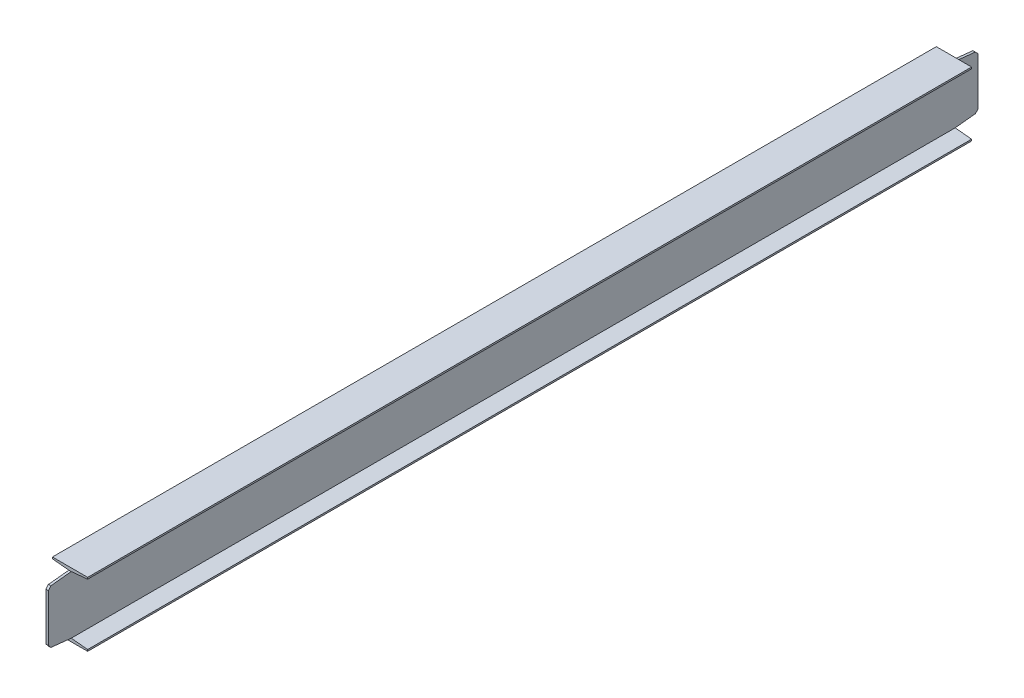
SolidWorks part; units mm, degrees
material "A3"
ref_plane "前视基准面" through (0, 0, 0) normal (0, 0, 1) x (1, 0, 0)
ref_plane "上视基准面" through (0, 0, 0) normal (0, 1, 0) x (1, 0, 0)
ref_plane "右视基准面" through (0, 0, 0) normal (1, 0, 0) x (0, 0, -1)
sketch "草图1" plane through (0, 0, 0) normal (0, 0, 1) x (1, 0, 0)
  line L0 (0, 80) -> (0, -80) construction
  line L1 (9.8926, 0) -> (-9.8926, 0) construction
  line L2 (44, 80) -> (-44, 80)
  line L3 (-44, 80) -> (-44, 76)
  line L4 (-44, 76) -> (-3, 72)
  line L5 (-3, 72) -> (-3, -72)
  line L6 (3, 72) -> (3, -72)
  line L7 (44, 76) -> (3, 72)
  line L8 (44, 80) -> (44, 76)
  line L9 (44, -80) -> (44, -76)
  line L10 (44, -76) -> (3, -72)
  line L11 (-44, -76) -> (-3, -72)
  line L12 (-44, -80) -> (-44, -76)
  line L13 (44, -80) -> (-44, -80)
  point P15 (0, 0)
  point P18 (3, 0)
  point P19 (-3, 0)
  dimension "D1" = 44
  dimension "D2" = 6
  dimension "D3" = 160
  dimension "D4" = 4
  dimension "D5" = 144
extrude "凸台-拉伸1" add sketch "草图1" along normal mid plane 2320
sketch "草图3" plane through (0, 0, 0) normal (1, 0, 0) x (0, 0, -1)
  line L0 (-1160, 66) -> (-1103, 72)
  line L1 (-1160, -72) -> (-1160, 72) construction
  line L2 (-1160, 72) -> (1160, 72) construction
  line L3 (-1103, 72) -> (-1103, 80)
  line L4 (-1160, 80) -> (1160, 80) construction
  line L5 (-1103, 80) -> (-1160, 80)
  line L6 (-1160, 80) -> (-1160, 66)
  line L7 (0, 0) -> (0, 80) construction
  line L8 (1160, 80) -> (1160, 66)
  line L9 (1103, 80) -> (1160, 80)
  line L10 (1103, 72) -> (1103, 80)
  line L11 (1160, 66) -> (1103, 72)
  line L12 (0, 0) -> (1160, 0) construction
  line L13 (1160, -72) -> (1160, 72) construction
  line L14 (1160, -66) -> (1103, -72)
  line L15 (1103, -72) -> (1103, -80)
  line L16 (1103, -80) -> (1160, -80)
  line L17 (1160, -80) -> (1160, -66)
  line L18 (-1160, -80) -> (-1160, -66)
  line L19 (-1103, -80) -> (-1160, -80)
  line L20 (-1103, -72) -> (-1103, -80)
  line L21 (-1160, -66) -> (-1103, -72)
  dimension "D1" = 57
  dimension "D2" = 66
extrude "切除-拉伸1" cut sketch "草图3" against normal through all both and the other way through all
chamfer "倒角1" distance 6 angle 45 4 edges at (0, -66, -1160) (0, 66, -1160) (0, -66, 1160) (0, 66, 1160)
